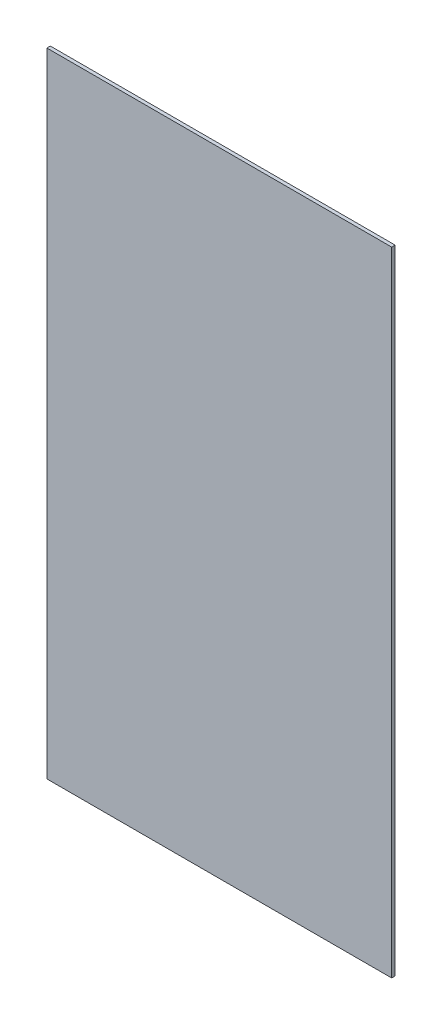
SolidWorks part; units mm, degrees
material "PMMA(有机玻璃)"
ref_plane "前视" through (0, 0, 0) normal (0, 0, 1) x (1, 0, 0)
ref_plane "上视" through (0, 0, 0) normal (0, 1, 0) x (1, 0, 0)
ref_plane "右视" through (0, 0, 0) normal (1, 0, 0) x (0, 0, -1)
sketch "草图1" plane through (0, 0, 0) normal (0, 0, 1) x (1, 0, 0)
  line L1 (-249.5, 458) -> (249.5, 458)
  line L2 (-249.5, 458) -> (-249.5, -458)
  line L3 (-249.5, -458) -> (249.5, -458)
  line L4 (249.5, 458) -> (249.5, -458)
  line L5 (-249.5, 458) -> (249.5, -458) construction
  line L6 (-249.5, -458) -> (249.5, 458) construction
  point P0 (0, 0)
  dimension "D1" = 916
  dimension "D2" = 499
extrude "凸台-拉伸1" add sketch "草图1" along normal blind 5
hole_wizard "M5 间隙孔1" positions "草图3" profile "草图2" hole size "M5" standard "GB"
sketch "草图3" plane through (0, 0, 5) normal (0, 0, 1) x (1, 0, 0)
  line L0 (-427.5, 273) -> (-427.5, -273) construction
  line L1 (-427.5, -273) -> (427.5, -273) construction
  line L2 (0, 273) -> (0, -273) construction
  line L3 (427.5, 273) -> (-427.5, 273) construction
  line L5 (-427.5, 0) -> (427.5, 0) construction
  line L6 (427.5, -273) -> (427.5, 273) construction
  point P0 (-375, -261)
  point P46 (415.5, 250)
  point P48 (-415.5, 250)
  point P58 (-125, -261)
  point P59 (125, -261)
  point P61 (-125, 261)
  point P62 (125, 261)
  point P64 (-375, 261)
  point P88 (375, -261)
  point P89 (375, 261)
  point P108 (415.5, 0)
  point P109 (-415.5, 0)
  point P110 (415.5, -250)
  point P111 (-415.5, -250)
  dimension "D1" = 12
  dimension "D2" = 12
  dimension "D5" = 3
  dimension "D3" = 12
  dimension "D6" = 4
  dimension "D4" = 2
sketch "草图2" plane through (-375, -261, 5) normal (1, 0, 0) x (0, -1, 0)
  line L0 (0, 0) -> (0, 5)
  line L1 (0, 5) -> (2.75, 5)
  line L2 (2.75, 5) -> (2.75, 0)
  line L5 (2.75, 0) -> (0, 0)
  line L11 (0, -6.35) -> (0, 107.95) construction
  dimension "通孔孔直径" = 5.5
  dimension "通孔孔深度" = 5
